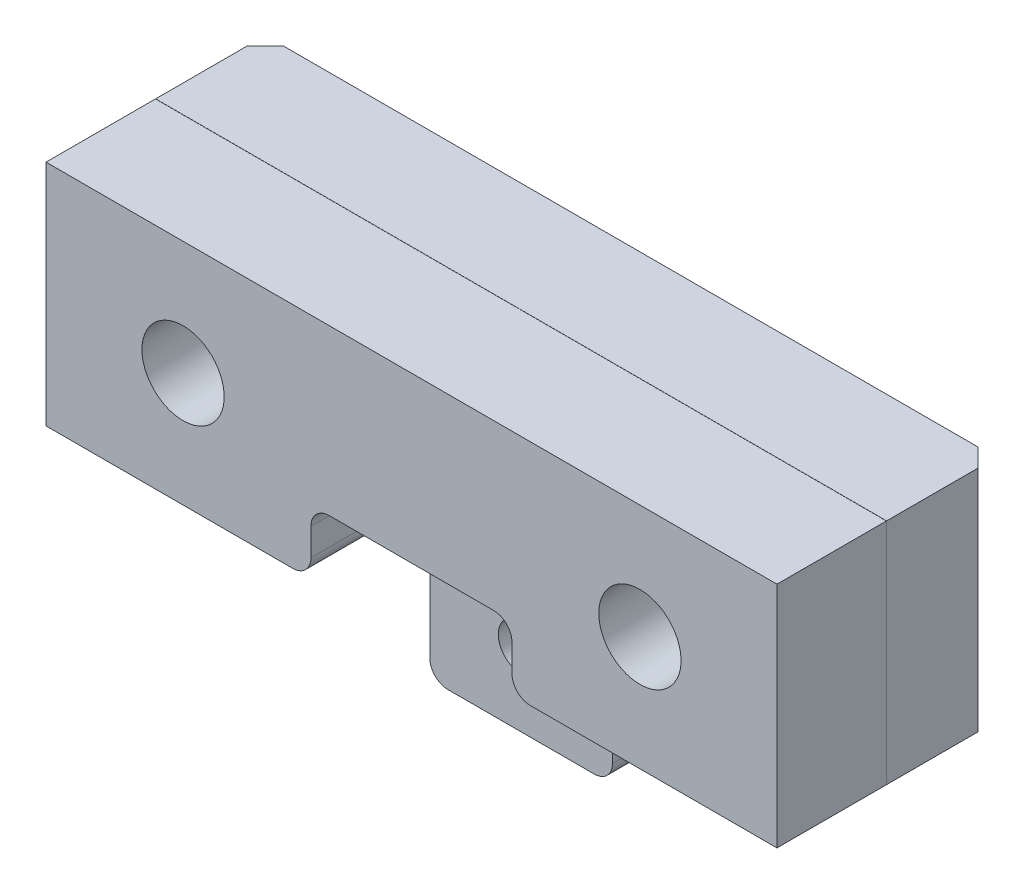
SolidWorks part; units mm, degrees
material "Q235"
ref_plane "Front Plane" through (0, 0, 0) normal (0, 0, 1) x (1, 0, 0)
ref_plane "Top Plane" through (0, 0, 0) normal (0, 1, 0) x (1, 0, 0)
ref_plane "Right Plane" through (0, 0, 0) normal (1, 0, 0) x (0, 0, -1)
sketch "Sketch1" plane through (0, 0, 0) normal (0, 1, 0) x (1, 0, 0)
  line L3 (80, 0) -> (80, 24)
  line L4 (80, 24) -> (0, 24)
  line L5 (0, 24) -> (0, 0)
  line L8 (40, 24) -> (40, 0) construction
  line L9 (0, 0) -> (80, 0)
  dimension "D1" = 24
  dimension "D4" = 80
extrude "Boss-Extrude1" add sketch "Sketch1" along normal mid plane 40
chamfer "Chamfer1" distance 2 angle 45 2 edges at (0, 0, -24) (80, 0, -24)
sketch "Sketch9" plane through (0, 0, 0) normal (0, 0, 1) x (1, 0, 0)
  line L0 (0, -20) -> (80, -20) construction
  line L1 (40, 20) -> (40, -5) construction
  line L2 (0, 20) -> (80, 20) construction
  line L12 (30, -5) -> (50, -5)
  line L13 (30, -5) -> (30, -20)
  line L14 (30, -20) -> (50, -20)
  line L15 (50, -5) -> (50, -20)
  dimension "D1" = 25
  dimension "D2" = 20
extrude "Cut-Extrude1" cut sketch "Sketch9" against normal blind 12
hole_wizard "M6 Tapped Hole1" positions "Sketch10" profile "Sketch11" tap size "M6" standard "GB"
sketch "Sketch10" plane through (0, 0, -24) normal (0, 0, -1) x (-1, 0, 0)
  line L0 (-40, 20) -> (-40, -12) construction
  line L1 (-78, 20) -> (-2, 20) construction
  line L4 (-78, -20) -> (-2, -20) construction
  point P0 (-40, -12)
  dimension "D1" = 8
sketch "Sketch11" plane through (40, -12, -24) normal (1, 0, 0) x (0, 1, 0)
  line L0 (0, 0) -> (0, 16.5022)
  line L1 (0, 16.5022) -> (2.5, 15)
  line L2 (2.5, 15) -> (2.5, 0)
  line L5 (2.5, 0) -> (0, 0)
  line L10 (0, 16.5022) -> (-2.5, 15) construction
  line L11 (0, -6.35) -> (0, 107.95) construction
  dimension "螺纹孔钻头直径" = 5
  dimension "螺纹孔钻头深度" = 15
  dimension "导头角度" = 118
cosmetic thread "Cosmetic Thread 5" parameters "D1"=12, "D2"=6
hole_wizard "M8 Clearance Hole1" positions "Sketch14" profile "Sketch15" hole size "M8" standard "GB"
sketch "Sketch14" plane through (0, 0, -24) normal (0, 0, -1) x (-1, 0, 0)
  line L0 (-40, 20) -> (-40, -20) construction
  line L1 (-78, 20) -> (-2, 20) construction
  line L2 (-78, -20) -> (-2, -20) construction
  line L4 (-40, 7.5) -> (-15, 7.5) construction
  point P0 (-65, 7.5)
  point P2 (-15, 7.5)
  dimension "D1" = 50
  dimension "D2" = 12.5
sketch "Sketch15" plane through (65, 7.5, -24) normal (1, 0, 0) x (0, 1, 0)
  line L0 (0, 0) -> (0, 32.7039)
  line L1 (0, 32.7039) -> (4.5, 30)
  line L2 (4.5, 30) -> (4.5, 0)
  line L5 (4.5, 0) -> (0, 0)
  line L10 (0, 32.7039) -> (-4.5, 30) construction
  line L11 (0, -6.35) -> (0, 107.95) construction
  dimension "孔直径" = 9
  dimension "孔深度" = 30
  dimension "导头角度" = 118
sketch "Sketch16" plane through (0, 0, -24) normal (0, 0, -1) x (-1, 0, 0)
  line L0 (-40, 20) -> (-40, -20) construction
  line L1 (-80, -20) -> (-50, -20)
  line L2 (-80, -20) -> (-80, -5)
  line L3 (-80, -5) -> (-50, -5)
  line L4 (-50, -20) -> (-50, -5)
  line L5 (-78, 20) -> (-2, 20) construction
  line L6 (-78, -20) -> (-2, -20) construction
  line L7 (-30, -20) -> (-30, -5)
  line L8 (0, -5) -> (-30, -5)
  line L9 (0, -20) -> (0, -5)
  line L10 (0, -20) -> (-30, -20)
  point P15 (-30, -12.5)
  dimension "D1" = 20
  dimension "D2" = 25
extrude "Cut-Extrude2" cut sketch "Sketch16" against normal through all
fillet "Fillet1" radius 5 2 edges at (50, -5, -18) (30, -5, -18)
fillet "Fillet2" radius 2 2 edges at (50, -20, -18) (30, -20, -18)
sketch "Sketch17" plane through (0, 0, 0) normal (0, 0, 1) x (1, 0, 0)
  line L0 (80, -5) -> (0, -5) construction
  line L1 (29, -5) -> (51, -5)
  line L2 (29, -5) -> (29, 2)
  line L3 (29, 2) -> (51, 2)
  line L4 (51, -5) -> (51, 2)
  line L5 (40, 20) -> (40, 2) construction
  line L6 (0, 20) -> (80, 20) construction
  dimension "D1" = 22
  dimension "D2" = 18
extrude "Cut-Extrude3" cut sketch "Sketch17" against normal blind 12
sketch "Sketch18" plane through (0, -5, 0) normal (0, -1, 0) x (1, 0, 0)
  line L0 (0, 0) -> (0, -22) construction
  line L1 (0, -11.98) -> (80, -11.98)
  line L2 (0, -11.98) -> (0, -12)
  line L3 (0, -12) -> (80, -12)
  line L4 (80, -11.98) -> (80, -12)
  line L5 (80, 0) -> (80, -22) construction
  line L6 (29, 0) -> (0, 0) construction
  dimension "D1" = 11.98
  dimension "D2" = 0.02
extrude "Cut-Extrude4" cut sketch "Sketch18" against normal through all
fillet "Fillet3" radius 2 4 edges at (51, 2, -5.99) (51, -5, -5.99) (29, 2, -5.99) (29, -5, -5.99)
sketch "Sketch19" plane through (0, 0, 0) normal (0, 0, 1) x (1, 0, 0)
  line L0 (66.5, -5) -> (66.5, -3) construction
  line L1 (80, -5) -> (53, -5) construction
  line L2 (56.5, -5) -> (56.5, -3)
  line L3 (76.5, -5) -> (76.5, -3)
  arc A0 (56.5, -5) -> (76.5, -5) centre (66.5, -5) ccw
  arc A1 (76.5, -3) -> (56.5, -3) centre (66.5, -3) ccw
  point P4 (66.5, -4)
  dimension "D1" = 20
  dimension "D2" = 2
extrude "Cut-Extrude5" [suppressed] cut sketch "Sketch19" against normal blind 10
